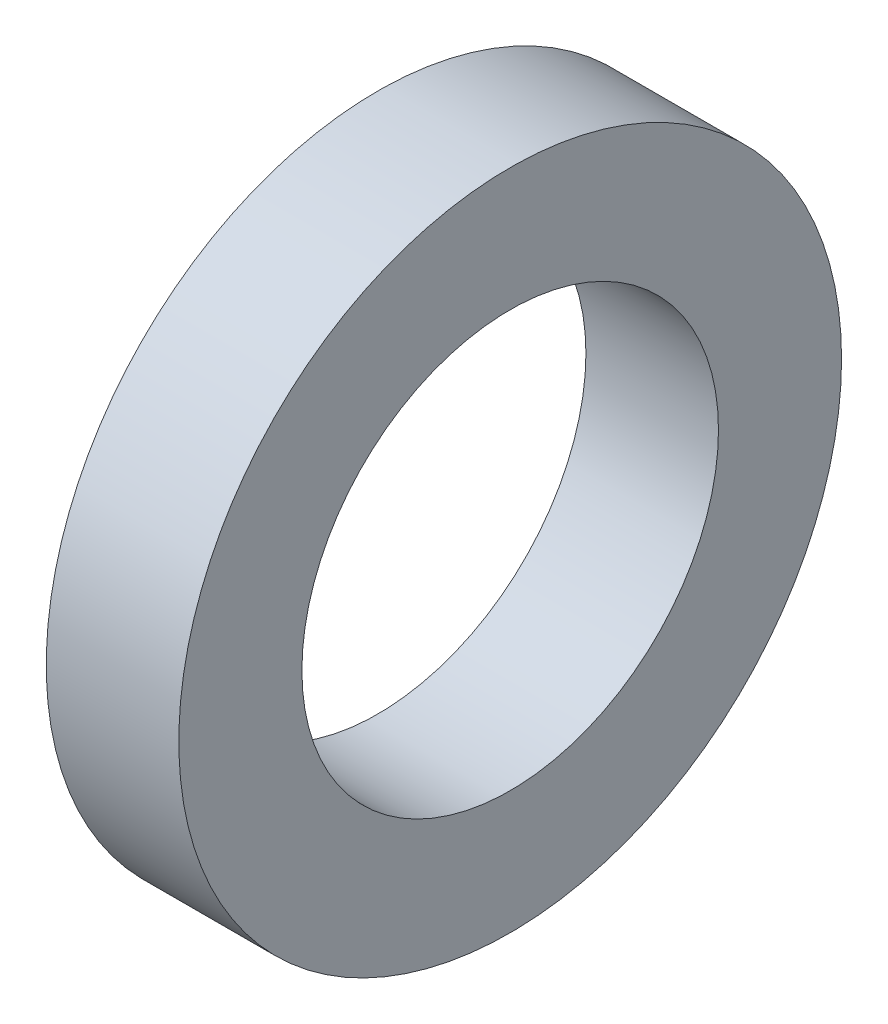
SolidWorks part; units mm, degrees
material "合金钢"
ref_plane "前视基准面" through (0, 0, 0) normal (0, 0, 1) x (1, 0, 0)
ref_plane "上视基准面" through (0, 0, 0) normal (0, 1, 0) x (1, 0, 0)
ref_plane "右视基准面" through (0, 0, 0) normal (1, 0, 0) x (0, 0, -1)
other "Configuration Table"
sketch "草图1" plane through (0, 0, 0) normal (1, 0, 0) x (0, 0, -1)
  circle A0 centre (0, 0) radius 11
  circle A1 centre (0, 0) radius 17.5
  dimension "D1" = 35
  dimension "D2" = 22
extrude "凸台-拉伸1" add sketch "草图1" along normal blind 7
